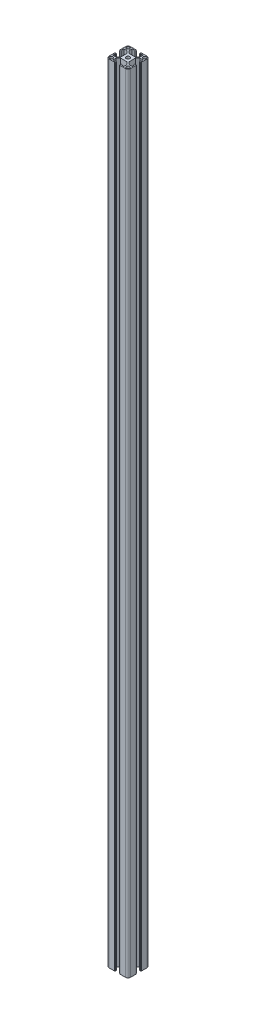
from build123d import *

# Parameters (mm, degrees)
SKETCH16_R     = 3.4
SKETCH16_R_2   = 3
MEMBER_1_DEPTH = 1467


with BuildPart() as part:
    # Sketch16 → Member 1 (new body)
    with BuildSketch(Plane(origin=(0, 0, 0), x_dir=(-1, 0, 0), z_dir=(0, 1, 0))):
        with BuildLine():
            Line((-5.1, 20), (-5.1, 19.5))
            Line((-5.1, 19.5), (-4.1, 19.5))
            Line((-4.1, 19.5), (-4.1, 17))
            Line((-4.1, 17), (-6.1, 17))
            Line((-6.1, 17), (-6.1, 18))
            Line((-6.1, 18), (-10.3, 18))
            Line((-10.3, 18), (-10.3, 12))
            Line((-10.3, 12), (-6, 7.7))
            Line((-6, 7.7), (6, 7.7))
            Line((6, 7.7), (10.3, 12))
            Line((10.3, 12), (10.3, 18))
            Line((10.3, 18), (6.1, 18))
            Line((6.1, 18), (6.1, 17))
            Line((6.1, 17), (4.1, 17))
            Line((4.1, 17), (4.1, 19.5))
            Line((4.1, 19.5), (5.1, 19.5))
            Line((5.1, 19.5), (5.1, 20))
            Line((5.1, 20), (15.5, 20))
            ThreePointArc((15.5, 20), (18.681980515, 18.681980515), (20, 15.5))
            Line((20, 15.5), (20, 5.1))
            Line((20, 5.1), (19.5, 5.1))
            Line((19.5, 5.1), (19.5, 4.1))
            Line((19.5, 4.1), (17, 4.1))
            Line((17, 4.1), (17, 6.1))
            Line((17, 6.1), (18, 6.1))
            Line((18, 6.1), (18, 10.3))
            Line((18, 10.3), (12, 10.3))
            Line((12, 10.3), (7.7, 6))
            Line((7.7, 6), (7.7, -6))
            Line((7.7, -6), (12, -10.3))
            Line((12, -10.3), (18, -10.3))
            Line((18, -10.3), (18, -6.1))
            Line((18, -6.1), (17, -6.1))
            Line((17, -6.1), (17, -4.1))
            Line((17, -4.1), (19.5, -4.1))
            Line((19.5, -4.1), (19.5, -5.1))
            Line((19.5, -5.1), (20, -5.1))
            Line((20, -5.1), (20, -15.5))
            ThreePointArc((20, -15.5), (18.681980515, -18.681980515), (15.5, -20))
            Line((15.5, -20), (5.1, -20))
            Line((5.1, -20), (5.1, -19.5))
            Line((5.1, -19.5), (4.1, -19.5))
            Line((4.1, -19.5), (4.1, -17))
            Line((4.1, -17), (6.1, -17))
            Line((6.1, -17), (6.1, -18))
            Line((6.1, -18), (10.3, -18))
            Line((10.3, -18), (10.3, -12))
            Line((10.3, -12), (6, -7.7))
            Line((6, -7.7), (-6, -7.7))
            Line((-6, -7.7), (-10.3, -12))
            Line((-10.3, -12), (-10.3, -18))
            Line((-10.3, -18), (-6.1, -18))
            Line((-6.1, -18), (-6.1, -17))
            Line((-6.1, -17), (-4.1, -17))
            Line((-4.1, -17), (-4.1, -19.5))
            Line((-4.1, -19.5), (-5.1, -19.5))
            Line((-5.1, -19.5), (-5.1, -20))
            Line((-5.1, -20), (-15.5, -20))
            ThreePointArc((-15.5, -20), (-18.681980515, -18.681980515), (-20, -15.5))
            Line((-20, -15.5), (-20, -5.1))
            Line((-20, -5.1), (-19.5, -5.1))
            Line((-19.5, -5.1), (-19.5, -4.1))
            Line((-19.5, -4.1), (-17, -4.1))
            Line((-17, -4.1), (-17, -6.1))
            Line((-17, -6.1), (-18, -6.1))
            Line((-18, -6.1), (-18, -10.3))
            Line((-18, -10.3), (-12, -10.3))
            Line((-12, -10.3), (-7.7, -6))
            Line((-7.7, -6), (-7.7, 6))
            Line((-7.7, 6), (-12, 10.3))
            Line((-12, 10.3), (-18, 10.3))
            Line((-18, 10.3), (-18, 6.1))
            Line((-18, 6.1), (-17, 6.1))
            Line((-17, 6.1), (-17, 4.1))
            Line((-17, 4.1), (-19.5, 4.1))
            Line((-19.5, 4.1), (-19.5, 5.1))
            Line((-19.5, 5.1), (-20, 5.1))
            Line((-20, 5.1), (-20, 15.5))
            ThreePointArc((-20, 15.5), (-18.681980515, 18.681980515), (-15.5, 20))
            Line((-15.5, 20), (-5.1, 20))
        make_face()
        Circle(SKETCH16_R, mode=Mode.SUBTRACT)
        with Locations((-15.556349186, 15.556349186)):
            Circle(SKETCH16_R_2, mode=Mode.SUBTRACT)
        with Locations((15.556349186, 15.556349186)):
            Circle(SKETCH16_R_2, mode=Mode.SUBTRACT)
        with Locations((15.556349186, -15.556349186)):
            Circle(SKETCH16_R_2, mode=Mode.SUBTRACT)
        with Locations((-15.556349186, -15.556349186)):
            Circle(SKETCH16_R_2, mode=Mode.SUBTRACT)
    extrude(amount=MEMBER_1_DEPTH)


solid = part.part
